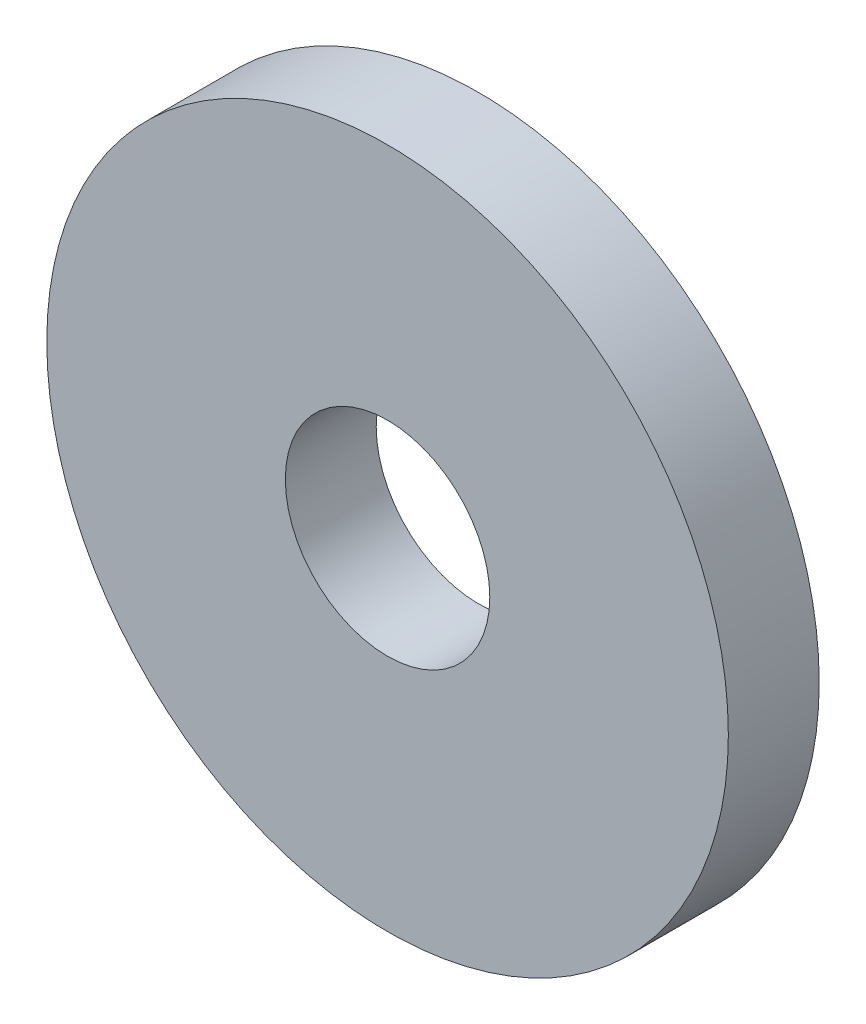
SolidWorks part; units mm, degrees
ref_plane "前视基准面" through (0, 0, 0) normal (0, 0, 1) x (1, 0, 0)
ref_plane "上视基准面" through (0, 0, 0) normal (0, 1, 0) x (1, 0, 0)
ref_plane "右视基准面" through (0, 0, 0) normal (1, 0, 0) x (0, 0, -1)
sketch "草图1" plane through (0, 0, 0) normal (0, 0, 1) x (1, 0, 0)
  circle A0 centre (0, 0) radius 7.5
  circle A1 centre (0, 0) radius 2.25
  dimension "D1" = 15
  dimension "D2" = 4.5
extrude "凸台-拉伸1" add sketch "草图1" along normal blind 2
